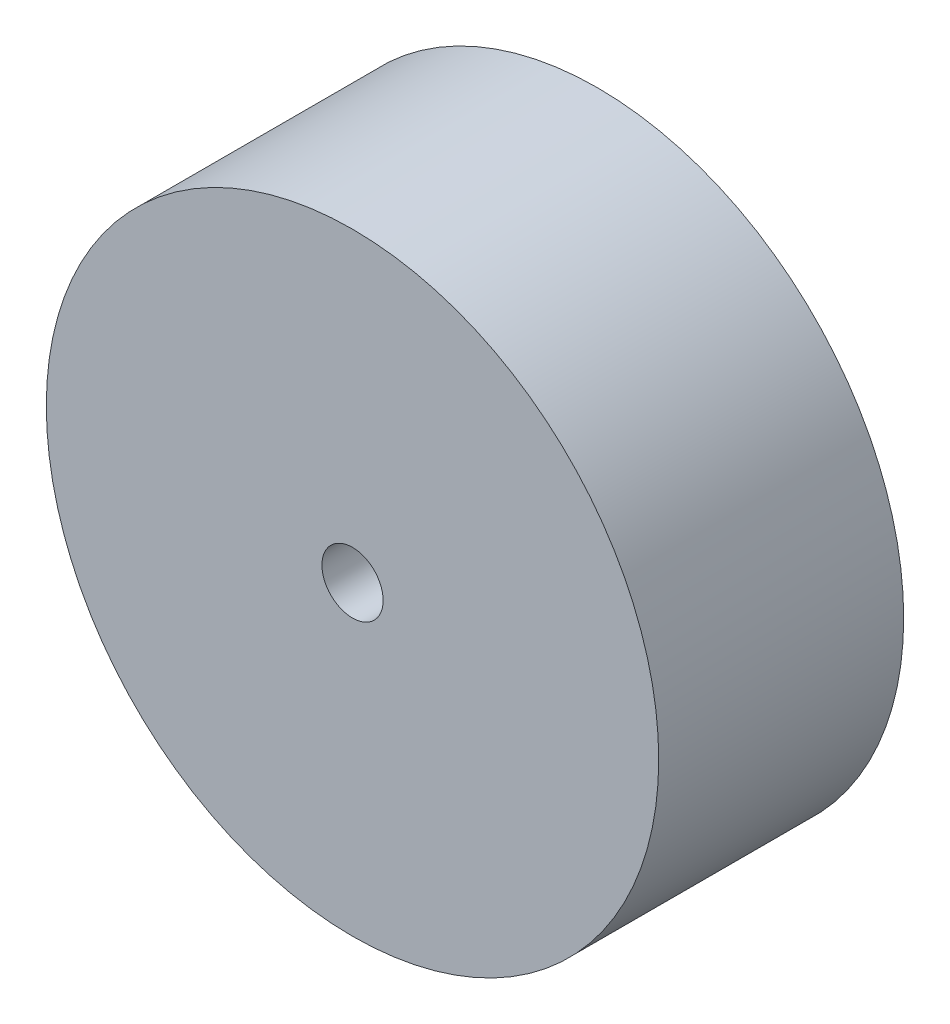
SolidWorks part; units mm, degrees
ref_plane "Front Plane" through (0, 0, 0) normal (0, 0, 1) x (1, 0, 0)
ref_plane "Top Plane" through (0, 0, 0) normal (0, 1, 0) x (1, 0, 0)
ref_plane "Right Plane" through (0, 0, 0) normal (1, 0, 0) x (0, 0, -1)
sketch "Sketch1" plane through (0, 0, 0) normal (0, 0, 1) x (1, 0, 0)
  circle A0 centre (0, 0) radius 15
  circle A1 centre (0, 0) radius 1.5
  dimension "D1" = 30
  dimension "D2" = 3
extrude "Boss-Extrude1" add sketch "Sketch1" along normal blind 12
